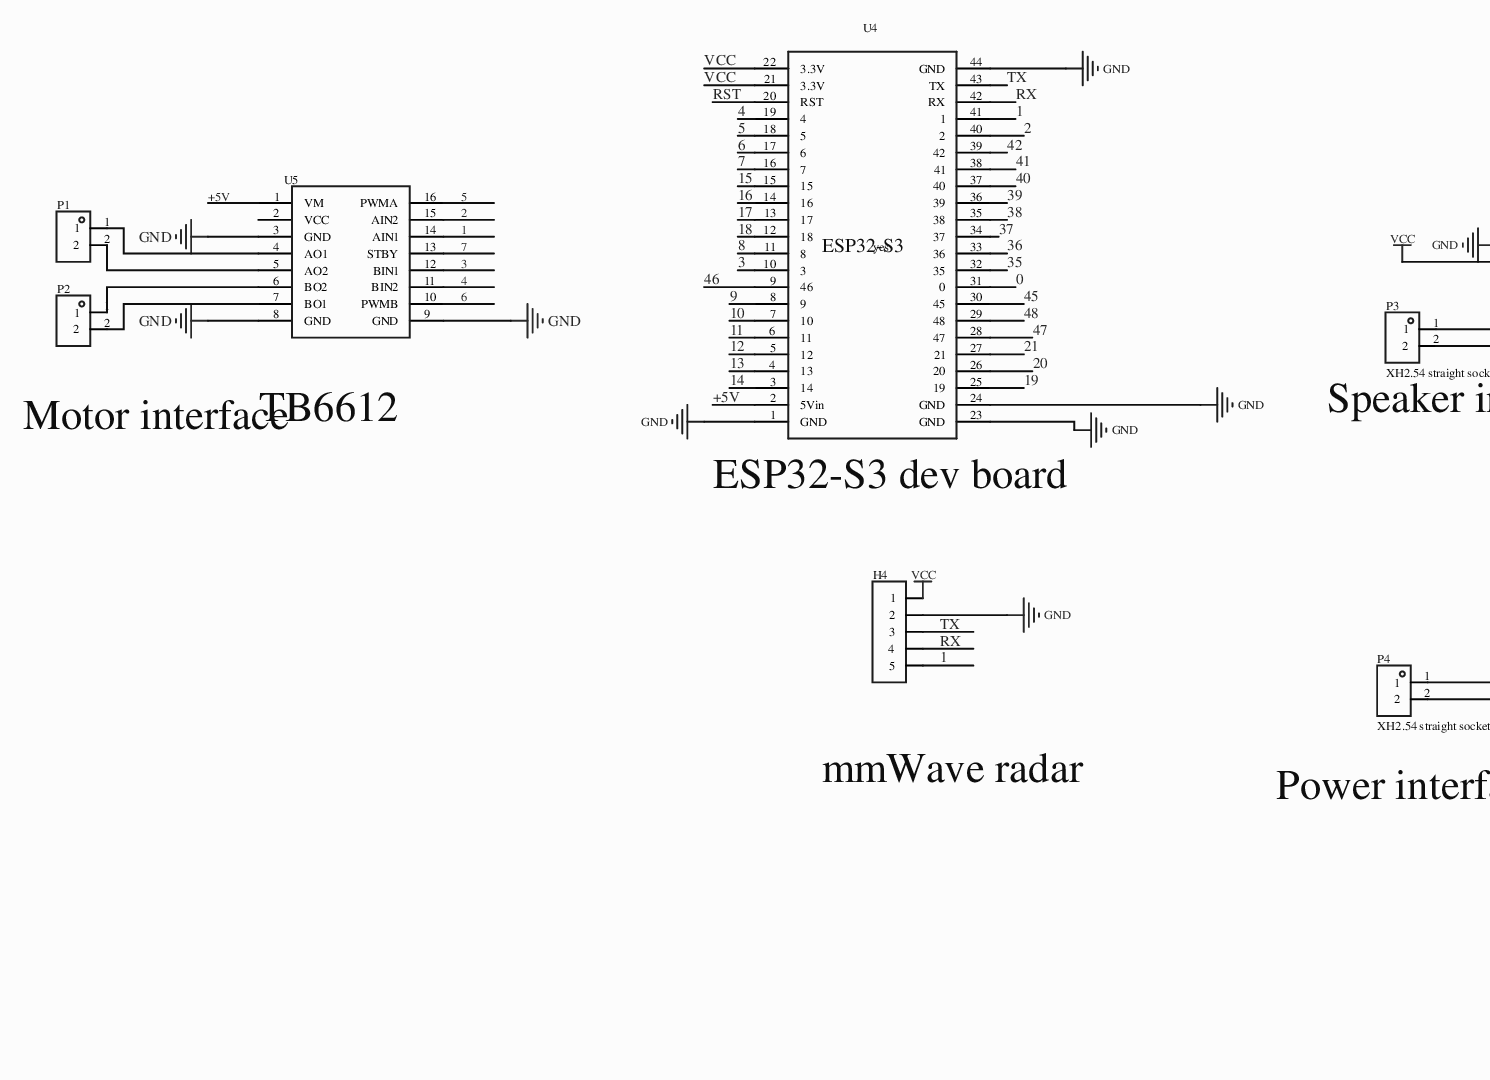
[diagram p0: MISC89096-3.schdoc, top left]
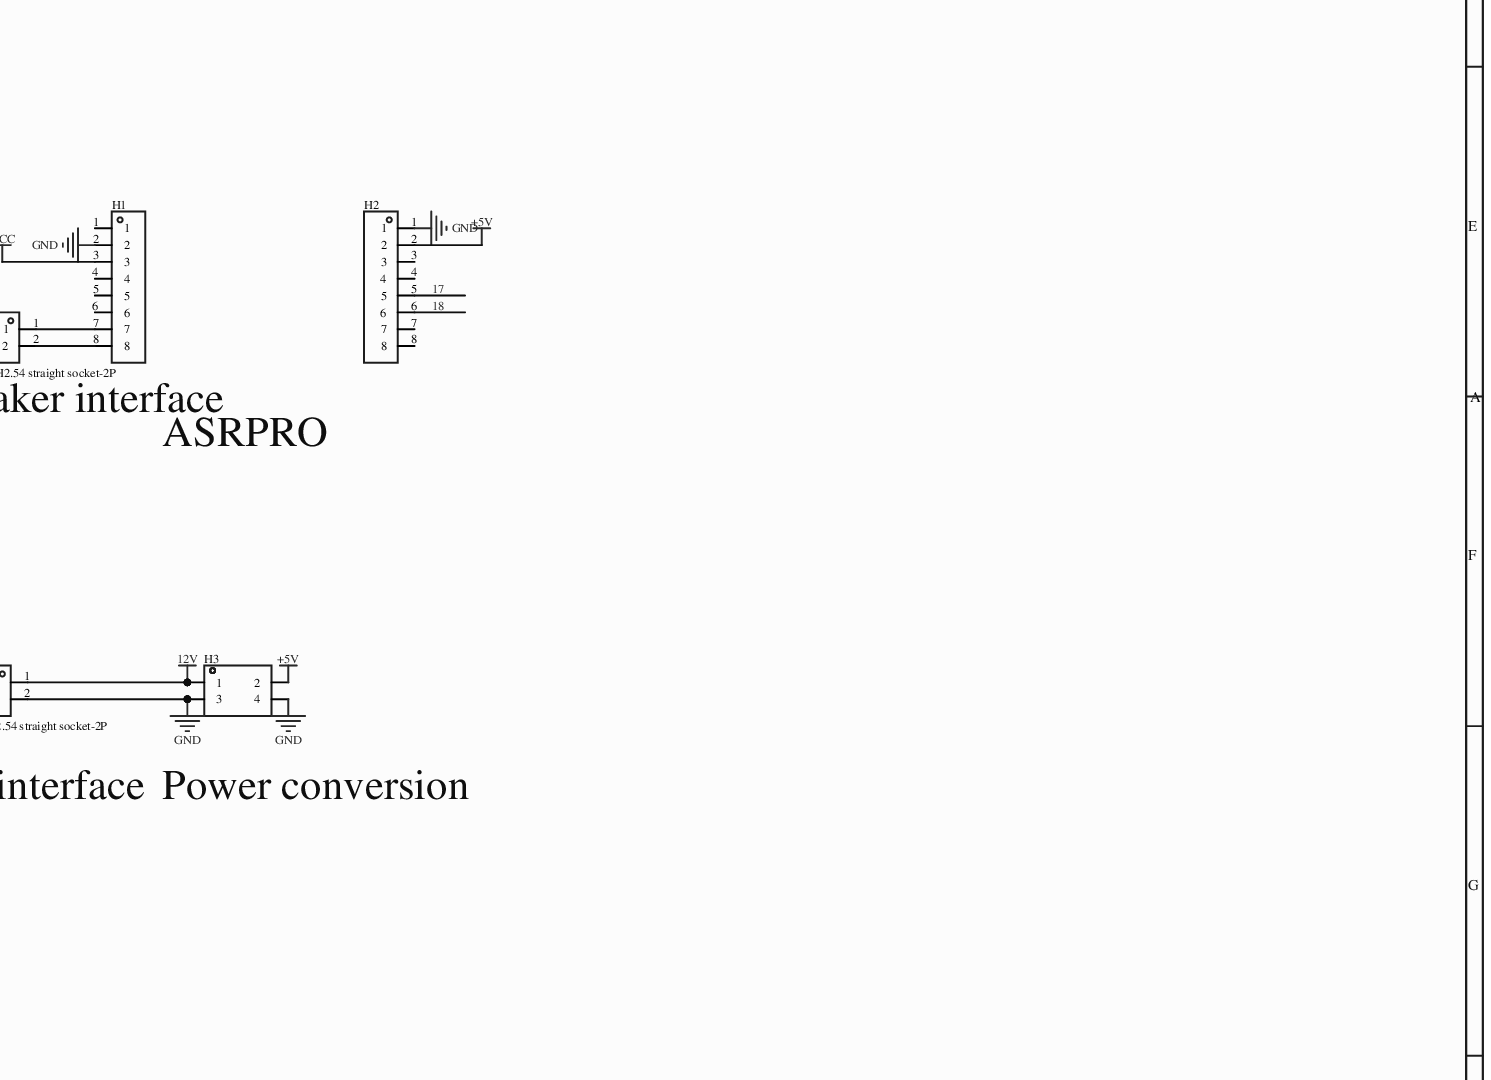
[diagram p1: MISC89096-3.schdoc, top right]
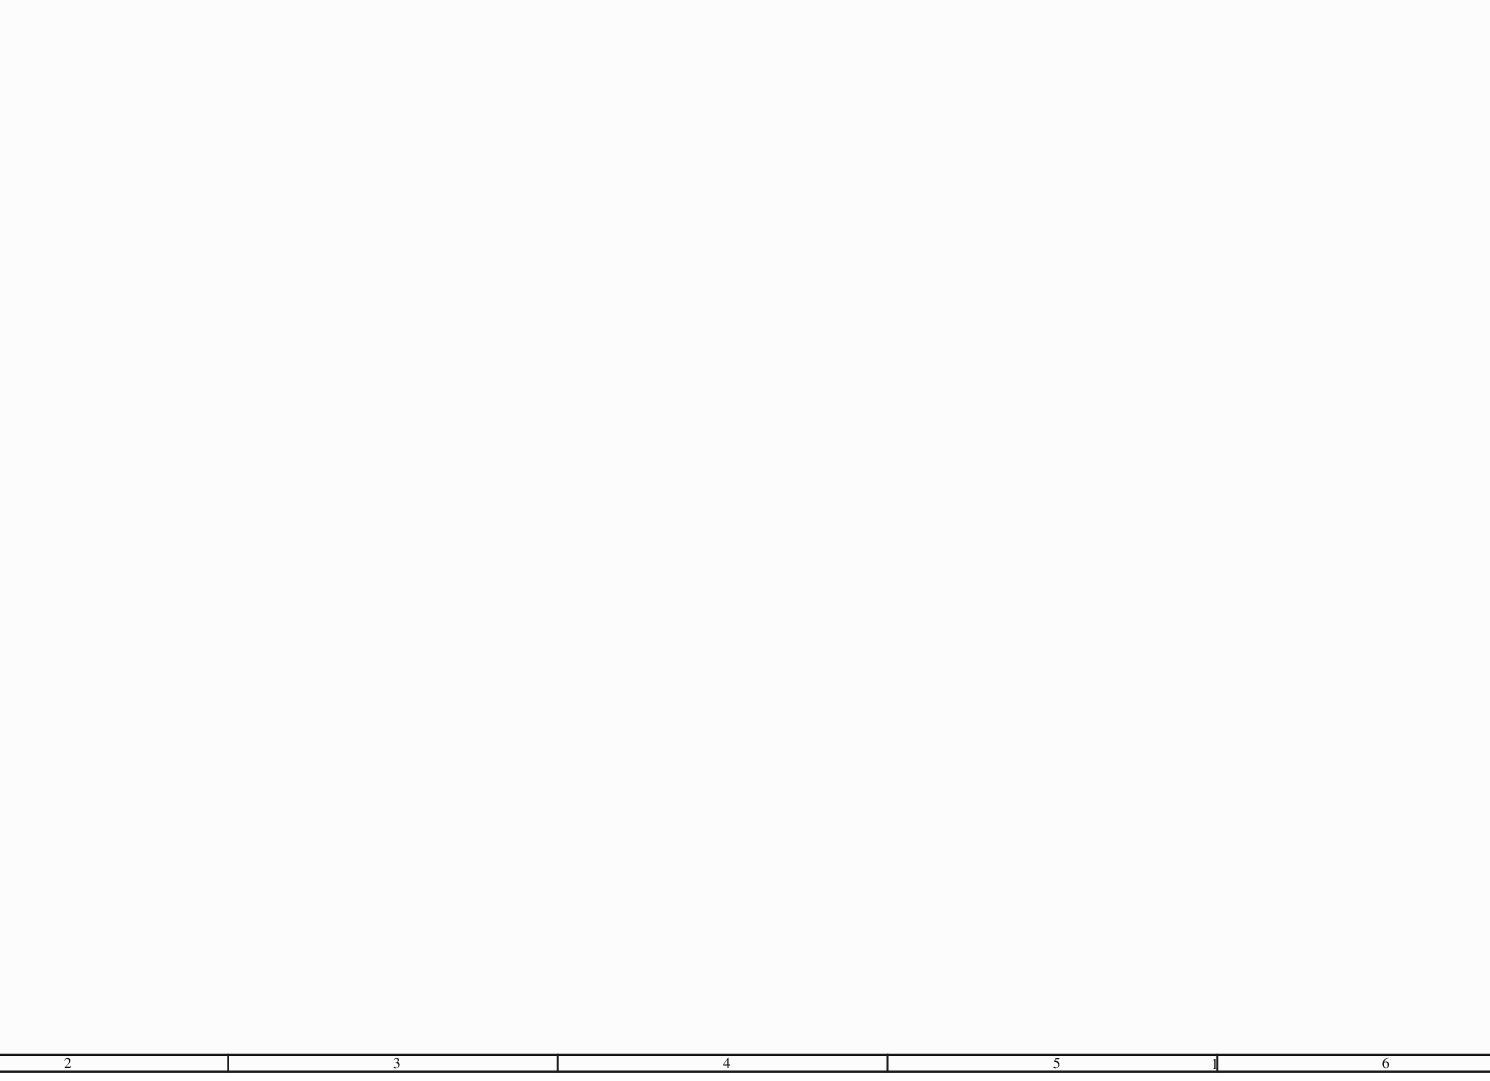
[diagram p2: MISC89096-3.schdoc, bottom left]
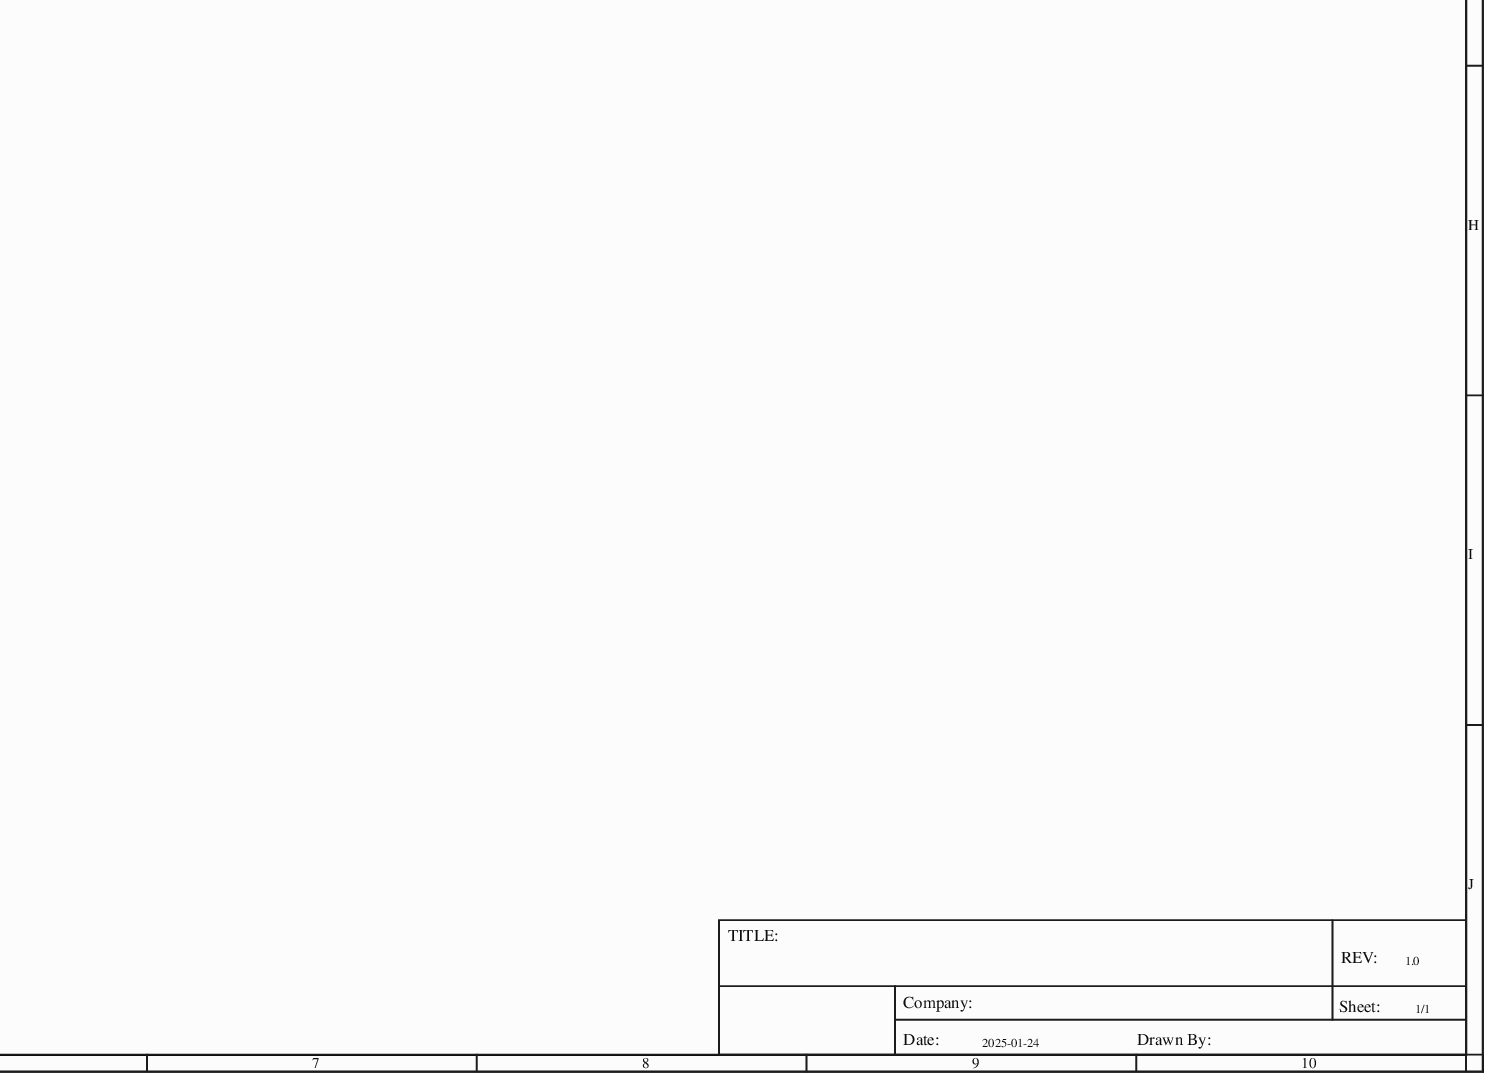
[diagram p3: MISC89096-3.schdoc, bottom right]
# Altium project MISC89096-2.PrjPcb
1 sheet, 10 parts. Net scope: global (net labels, ports and power ports of the same name join across sheets).
Board file: MISC89096.pcbdoc

## Sheet MISC89096-3.schdoc
size 503 x 503 mm; Name: MISC89096; @Project Name: MISC89096; REV: 1.0; Date: 2025-01-24; Sheet: 1/1; @Page No: 1; @Page Count: 1; @Schematic Name: MISC89096; @Board Name: MISC89096; @Update Date: 2026-04-14; @Create Time: 13:59:00; @Update Time: 16:32:12; @Create Date: 2026-04-14

### Parts
H1  (no value)  [HDR-TH_8P-P2.54-V-F-1]
H2  (no value)  [HDR-TH_8P-P2.54-V-F-1]
H3  (no value)  [HDR-TH_4P-P2.54-V-F-R2-C2-S2.54]
H4  (no value)  [HDR-TH_5P-P2.54-V-F]
P1  KF301-2P terminal block  [CONN-TH_XY301V-A-5.0-2P]  (value not drawn)
P2  KF301-2P terminal block  [CONN-TH_XY301V-A-5.0-2P]  (value not drawn)
P3  XH2.54 straight socket-2P  [CONN-TH_XH2.54-2P]
P4  XH2.54 straight socket-2P  [CONN-TH_XH2.54-2P]
U4  Add into BOM: yes  [ESP32S3]  (hidden comment: NO)
U5  (no value)  [tb6612]

### Nets
12V: H3.1 P4.1
+5V: H2.2 H3.2 U4.2(5Vin) U5.1(VM)
GND: H1.2 H2.1 H3.3 H3.4 H4.2 P4.2 U4.1(GND) U4.23(GND) U4.24(GND) U4.44(GND) U5.3(GND) U5.8(GND) U5.9(GND)
VCC: H1.3 H4.1 U4.21(3.3V) U4.22(3.3V)
0: U4.31(0)
1: H4.5 U4.41(1) U5.14(AIN1)
2: U4.40(2) U5.15(AIN2)
3: U4.10(3) U5.12(BIN1)
4: U4.19(4) U5.11(BIN2)
5: U4.18(5) U5.16(PWMA)
6: U4.17(6) U5.10(PWMB)
7: U4.16(7) U5.13(STBY)
8: U4.11(8)
9: U4.8(9)
10: U4.7(10)
11: U4.6(11)
12: U4.5(12)
13: U4.4(13)
14: U4.3(14)
15: U4.15
16: U4.14(16)
17: H2.5 U4.13(17)
18: H2.6 U4.12(18)
19: U4.25(19)
20: U4.26(20)
21: U4.27(21)
35: U4.32(35)
36: U4.33(36)
37: U4.34(37)
38: U4.35(38)
39: U4.36(39)
40: U4.37(40)
41: U4.38(41)
42: U4.39(42)
45: U4.30(45)
46: U4.9(46)
47: U4.28(47)
48: U4.29(48)
RST: U4.20(RST)
RX: H4.4 U4.42(RX)
TX: H4.3 U4.43(TX)
NetH1_7: H1.7 P3.1
NetH1_8: H1.8 P3.2
NetP1_1: P1.1 U5.4(AO1)
NetP1_2: P1.2 U5.5(AO2)
NetP2_1: P2.1 U5.6(BO2)
NetP2_2: P2.2 U5.7(BO1)

Not connected (* = marked no-connect by the designer): H1 1 4 5 6; H2 3 4 7 8; U5 2(VCC)

### Notes on the sheet
- Speaker interface
- Motor interface
- (near U5) TB6612
- (near U4) ESP32-S3 dev board
- ASRPRO
- mmWave radar
- Power interface
- (near H3) Power conversion
- 1
- 2
- 3
- 4
- 5
- 6
- 7
- 8
- 9
- 10
- A
- B
- C
- D
- E
- F
- G
- H
- I
- J
- TITLE:
- Company:
- Sheet:
- REV:
- 1.0
- 1/1
- Date:
- 2025-01-24
- Drawn By:

### Library data of the parts
H1 H2 = HDR-F_2.54_1x8P: Symbol: Header-Female-2.54_1x8; AddInBom: yes; ModelId: 0f7e4d9227ef4fa08d5469c22cc70cdb0819f05c4eef4c71ace90d822a990e87; ModelName: HDR-F-2.54_1x8; ModelTransform: 799.99844,100,0,0,0,0,0,0,-118.11; Device: HDR-F_2.54_1x8P; ConvertToPcb: yes; FootprintName: HDR-TH_8P-P2.54-V-F-1; SupplierPart: C27438; Supplier Footprint: 插件
H3 = HDR-F_2.54_2x2: Symbol: HDR-F-2.54_2x2; ConvertToPcb: yes; ModelId: 870c884146ee4765973edc845f10b7af0819f05c4eef4c71ace90d822a990e87; ModelName: HDR-TH_4P-P2.54-F-LI-2X2P; ModelTransform: 215.7476,196.85,0,0,0,0,0,0,-118.11; Device: HDR-F_2.54_2x2; AddInBom: yes; SupplierPart: C92273; Supplier Footprint: 插件; FootprintName: HDR-TH_4P-P2.54-V-F-R2-C2-S2.54
H4 = HDR-F_2.54_1x5P: Symbol: Header-Female-2.54_1x5; ConvertToPcb: yes; ModelId: f49cb6116a3d45e5a64915bf3e00773f0819f05c4eef4c71ace90d822a990e87; ModelTransform: 519.684,98.464,0,0,0,0,0,0,-124.016; Device: HDR-F_2.54_1x5P; AddInBom: yes; SupplierPart: C50950; Supplier Footprint: 插件; FootprintName: HDR-TH_5P-P2.54-V-F; ModelName: HDR-TH_5P-P2.54-V-F
P1 P2 = KF301-2P接线端子: 3D Model: ef7ead88b0f2448d904975b26718870f; 3D Model Transform: 417.322,299.212,0,0,0,0,11.811,-7.835,-157.48; AddInBom: yes; Symbol: KF301-2P terminal block; Device: KF301-2P terminal block; LCSC Part Name: KF301-2P接线端子; Supplier Part: C9900016950; Manufacturer Part: KF301-2P接线端子; Supplier Footprint: CK301-2P; Supplier: LCSC; ConvertToPcb: yes; FootprintName: CONN-TH_XY301V-A-5.0-2P; ModelName: CONN-TH_XY301V-A-5.0-2P
P3 P4 = XH2.54直插座-2P: AddInBom: yes; ModelId: c3cc11bd8b8748c1ae6bc231aac3a1ff0819f05c4eef4c71ace90d822a990e87; ModelTransform: 296.889,230.315,0,0,0,0,0,26.653,-137.795; Symbol: XH2.54 straight socket-2P; Device: XH2.54 straight socket-2P; LCSC Part Name: XH2.54直插座-2P; SupplierPart: C9900016957; ManufacturerPart: XH2.54直插座-2P; Supplier Footprint: XH2.54-2; JLCPCB Part Class: Extended Part; Supplier: LCSC; ConvertToPcb: yes; FootprintName: CONN-TH_XH2.54-2P; ModelName: CONN-TH_XH2.54-2P
U5 = tb6612: AddInBom: yes; Symbol: tb6612; Device: tb6612; JLCPCB Part Class: Extended; ConvertToPcb: yes; FootprintName: tb6612
U4 = NO: Origin Footprint: ESP32S3; Device: NO; Symbol: NO; Convert to PCB: yes; FootprintName: ESP32S3